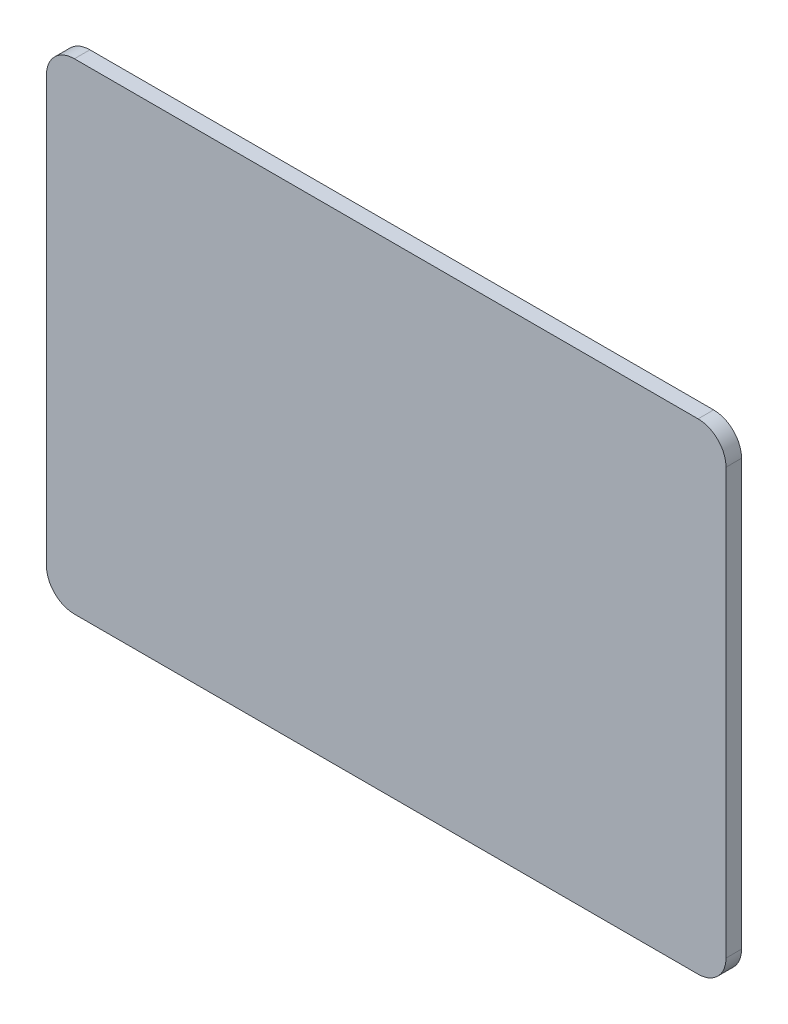
from build123d import *

# Parameters (mm, degrees)
SKETCH1_W           = 219
SKETCH1_H           = 155
BOSS_EXTRUDE1_DEPTH = 5
FILLET1_R           = 9


with BuildPart() as part:
    # Sketch1 → Boss-Extrude1 (new body)
    with BuildSketch(Plane.XY):
        with Locations((109.5, -77.5)):
            Rectangle(SKETCH1_W, SKETCH1_H)
    extrude(amount=BOSS_EXTRUDE1_DEPTH)

    # Fillet1
    fillet1_edges = [part.edges().sort_by_distance(p)[0] for p in [
        (0, 0, 2.5),
        (219, 0, 2.5),
        (219, -155, 2.5),
        (0, -155, 2.5),
    ]]
    fillet(fillet1_edges, radius=FILLET1_R)


solid = part.part
